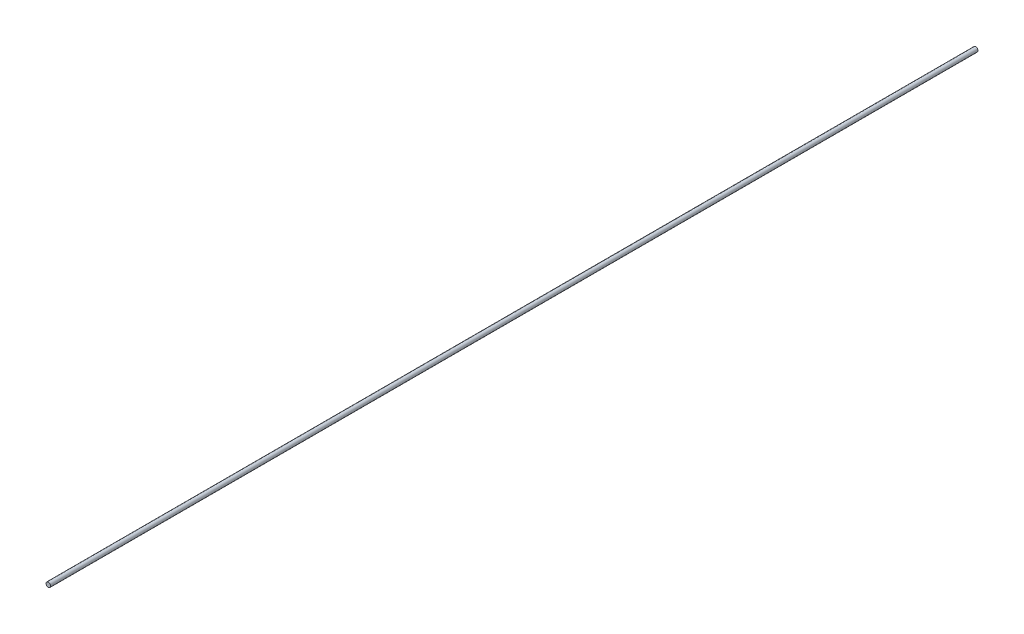
from build123d import *

# Parameters (mm, degrees)
SKETCH2_R           = 2
BOSS_EXTRUDE1_DEPTH = 810


with BuildPart() as part:
    # Sketch2 → Boss-Extrude1 (new body)
    with BuildSketch(Plane.XY):
        Circle(SKETCH2_R)
    extrude(amount=BOSS_EXTRUDE1_DEPTH)


solid = part.part
